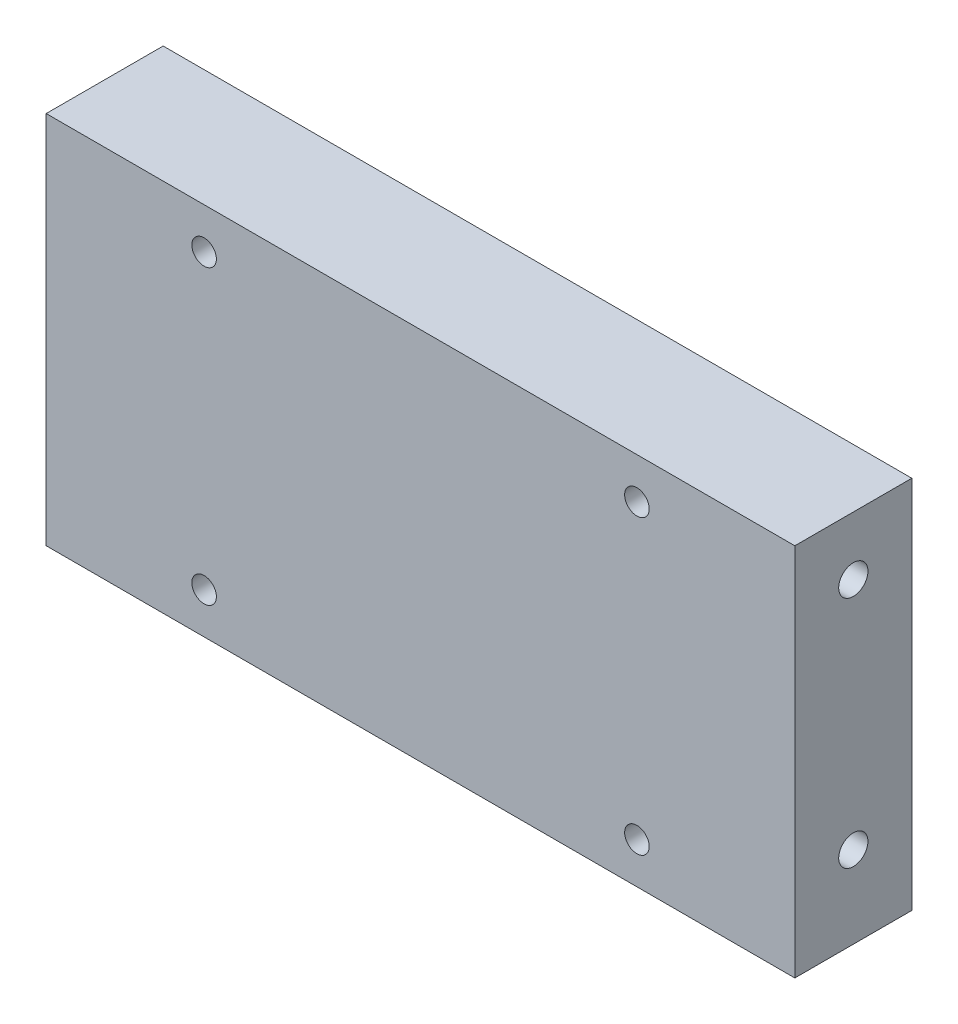
SolidWorks part; units mm, degrees
ref_plane "前视" through (0, 0, 0) normal (0, 0, 1) x (1, 0, 0)
ref_plane "上视" through (0, 0, 0) normal (0, 1, 0) x (1, 0, 0)
ref_plane "右视" through (0, 0, 0) normal (1, 0, 0) x (0, 0, -1)
sketch "草图1" plane through (0, 0, 0) normal (0, 0, 1) x (1, 0, 0)
  line L1 (0, 0) -> (128, 0)
  line L2 (0, 0) -> (0, 64)
  line L3 (0, 64) -> (128, 64)
  line L4 (128, 0) -> (128, 64)
  dimension "D1" = 64
  dimension "D2" = 128
extrude "拉伸1" add sketch "草图1" along normal blind 20
hole_wizard "M5 螺纹孔1" positions "草图3" profile "草图2" tap size "M5" standard "GB" end condition through all
sketch "草图3" plane through (0, 0, 20) normal (0, 0, 1) x (1, 0, 0)
  line L0 (64, 64) -> (64, 0) construction
  line L1 (128, 64) -> (0, 64) construction
  line L2 (0, 0) -> (128, 0) construction
  line L3 (0, 32) -> (160, 32) construction
  point P0 (27, 57)
  point P13 (27, 7)
  point P14 (101, 7)
  point P15 (101, 57)
  dimension "D1" = 50
  dimension "D2" = 37
  dimension "D3" = 32
sketch "草图2" plane through (27, 57, 20) normal (1, 0, 0) x (0, -1, 0)
  line L0 (0, 0) -> (0, 20)
  line L1 (0, 20) -> (2.1, 20)
  line L2 (2.1, 20) -> (2.1, 0)
  line L5 (2.1, 0) -> (0, 0)
  line L11 (0, -6.35) -> (0, 107.95) construction
  dimension "通孔螺纹孔钻头直径" = 4.2
  dimension "通孔螺纹孔钻头深度" = 20
cosmetic thread "孔螺蚊线1" parameters "D2"=5
cosmetic thread "孔螺蚊线2" parameters "D2"=5
cosmetic thread "孔螺蚊线3" parameters "D2"=5
cosmetic thread "孔螺蚊线4" parameters "D2"=5
hole_wizard "M5x0.8 螺纹孔1" positions "草图5" profile "草图4" tap size "M5x0.8" standard "Ansi Metric"
sketch "草图5" plane through (0, 0, 0) normal (-1, 0, 0) x (0, 0, 1)
  line L0 (10, 64) -> (10, 0) construction
  line L1 (20, 64) -> (0, 64) construction
  line L2 (20, 0) -> (0, 0) construction
  point P0 (10, 54)
  dimension "D1" = 10
sketch "草图4" plane through (0, 54, 10) normal (0, 1, 0) x (0, 0, 1)
  line L0 (0, 0) -> (0, 18.6618)
  line L1 (0, 18.6618) -> (2.1, 17.4)
  line L2 (2.1, 17.4) -> (2.1, 15)
  line L3 (2.1, 15) -> (2.5, 15)
  line L4 (2.5, 15) -> (2.5, 0)
  line L5 (2.5, 0) -> (0, 0)
  line L10 (0, 18.6618) -> (-2.1, 17.4) construction
  line L11 (0, -6.35) -> (0, 107.95) construction
  dimension "蹟恇謂郰芛眻噤" = 4.2
  dimension "蹟恇謂郰芛旮僅" = 17.4
  dimension "蹟恇翋眻噤" = 5
  dimension "蹟恇旮僅" = 15
  dimension "絳芛褒僅" = 118
ref_plane "基准面1" through (64, 0, 0) normal (1, 0, 0) x (0, 0, -1)
mirror "镜向1" about plane through (64, 0, 0) normal (1, 0, 0) of "M5x0.8 螺纹孔1"
pattern_linear "阵列(线性)1" count 2 spacing 40 along (0, -1, 0) of "M5x0.8 螺纹孔1"
mirror "镜向2" about plane through (64, 0, 0) normal (1, 0, 0) of "阵列(线性)1"
